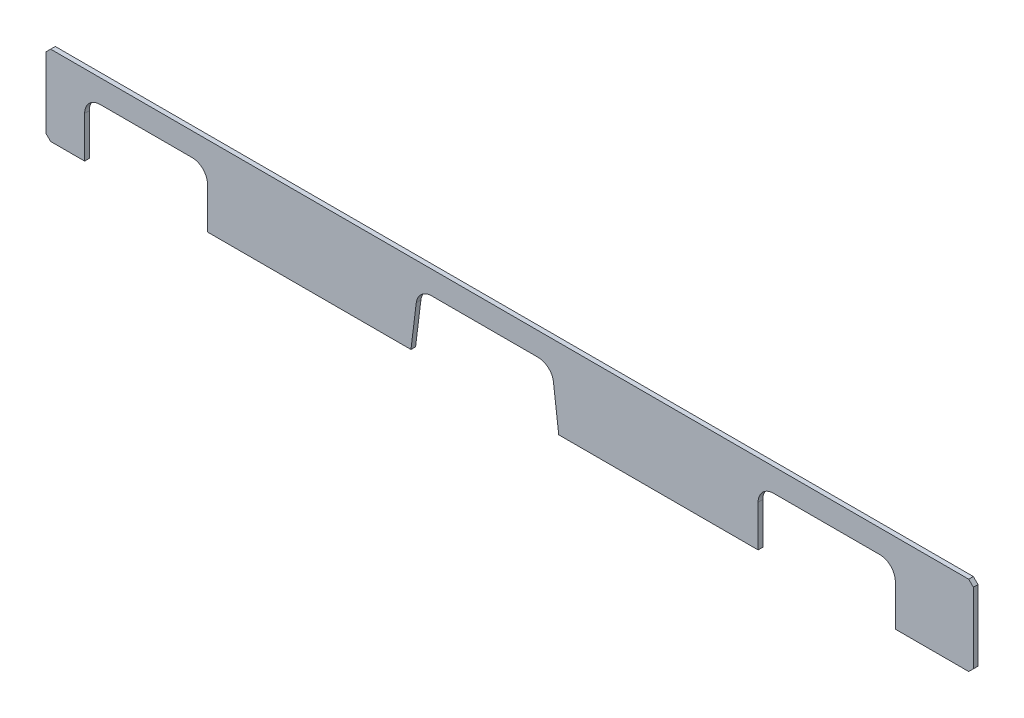
from build123d import *

# Parameters (mm, degrees)
BOSS_EXTRUDE1_DEPTH = 12


with BuildPart() as part:
    # Sketch1 → Boss-Extrude1 (new body)
    with BuildSketch(Plane.XY):
        with BuildLine():
            Line((140, 147), (378, 147))
            ThreePointArc((378, 147), (406.284271247, 135.284271247), (418, 107))
            Line((418, 107), (418, 0))
            Line((418, 0), (944.5, 0))
            Line((944.5, 0), (958.236494969, 111.874773736))
            ThreePointArc((958.236494969, 111.874773736), (971.433539106, 136.958228832), (997.938341035, 147))
            Line((997.938341035, 147), (1273.561658965, 147))
            ThreePointArc((1273.561658965, 147), (1300.066460894, 136.958228832), (1313.263505031, 111.874773736))
            Line((1313.263505031, 111.874773736), (1327, 0))
            Line((1327, 0), (1843, 0))
            Line((1843, 0), (1843, 107))
            ThreePointArc((1843, 107), (1854.715728753, 135.284271247), (1883, 147))
            Line((1883, 147), (2158, 147))
            ThreePointArc((2158, 147), (2186.284271247, 135.284271247), (2198, 107))
            Line((2198, 107), (2198, 0))
            Line((2198, 0), (2388, 0))
            Line((2388, 0), (2400, 12))
            Line((2400, 12), (2400, 195))
            Line((2400, 195), (2388, 207))
            Line((2388, 207), (12, 207))
            Line((12, 207), (0, 195))
            Line((0, 195), (0, 12))
            Line((0, 12), (12, 0))
            Line((12, 0), (100, 0))
            Line((100, 0), (100, 107))
            ThreePointArc((100, 107), (111.715728753, 135.284271247), (140, 147))
        make_face()
    extrude(amount=BOSS_EXTRUDE1_DEPTH)


solid = part.part
